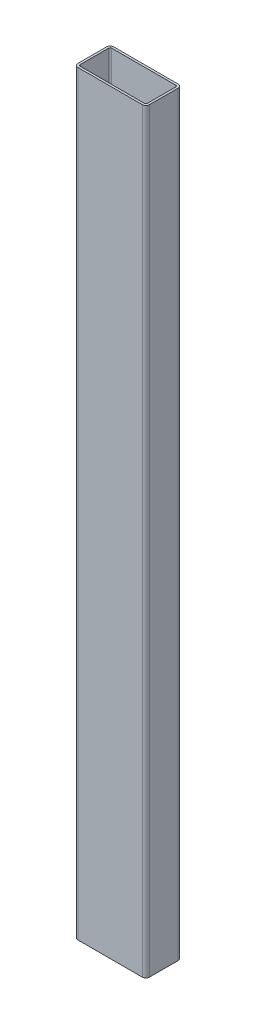
from build123d import *

# Parameters (mm, degrees)
EXTRUDE_THIN1_DEPTH = 1057


with BuildPart() as part:
    # Sketch1 → Extrude-Thin1 (new, symmetric)
    with BuildSketch(Plane(origin=(0, 0, 0), x_dir=(1, 0, 0), z_dir=(0, 1, 0))):
        with BuildLine():
            Line((-90, 50), (90, 50))
            ThreePointArc((90, 50), (97.071067812, 47.071067812), (100, 40))
            Line((100, 40), (100, -40))
            ThreePointArc((100, -40), (97.071067812, -47.071067812), (90, -50))
            Line((90, -50), (-90, -50))
            ThreePointArc((-90, -50), (-97.071067812, -47.071067812), (-100, -40))
            Line((-100, -40), (-100, 40))
            ThreePointArc((-100, 40), (-97.071067812, 47.071067812), (-90, 50))
        make_face()
        with BuildLine():
            Line((-90, 44), (90, 44))
            ThreePointArc((90, 44), (92.828427125, 42.828427125), (94, 40))
            Line((94, 40), (94, -40))
            ThreePointArc((94, -40), (92.828427125, -42.828427125), (90, -44))
            Line((90, -44), (-90, -44))
            ThreePointArc((-90, -44), (-92.828427125, -42.828427125), (-94, -40))
            Line((-94, -40), (-94, 40))
            ThreePointArc((-94, 40), (-92.828427125, 42.828427125), (-90, 44))
        make_face(mode=Mode.SUBTRACT)
    extrude(amount=EXTRUDE_THIN1_DEPTH, both=True)


solid = part.part
